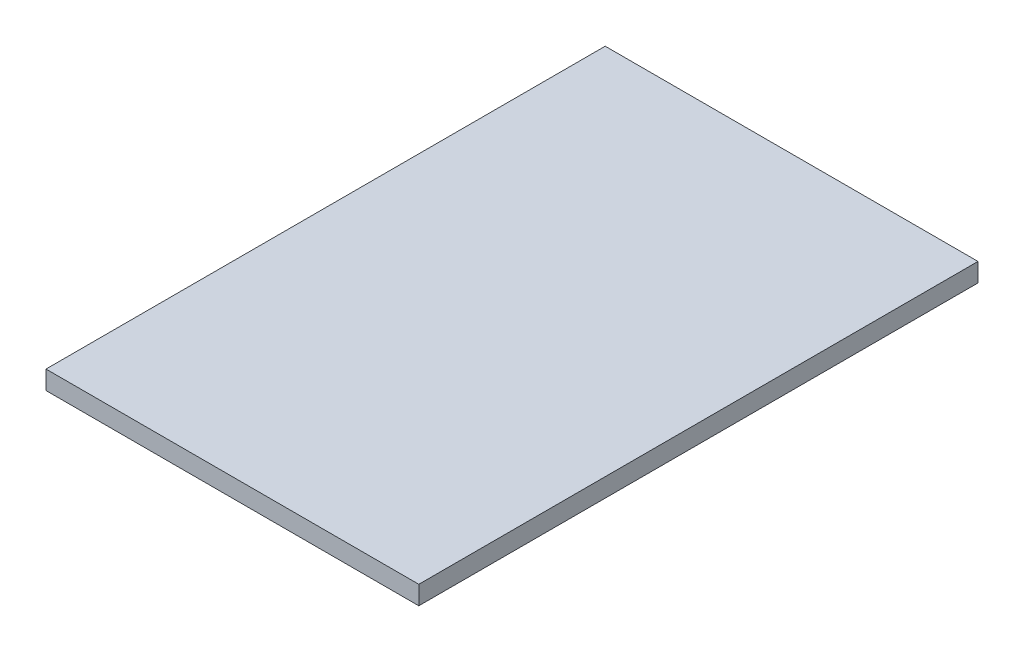
SolidWorks part; units mm, degrees
ref_plane "Front Plane" through (0, 0, 0) normal (0, 0, 1) x (1, 0, 0)
ref_plane "Top Plane" through (0, 0, 0) normal (0, 1, 0) x (1, 0, 0)
ref_plane "Right Plane" through (0, 0, 0) normal (1, 0, 0) x (0, 0, -1)
sketch "Sketch1" plane through (0, 0, 0) normal (0, 1, 0) x (1, 0, 0)
  line L1 (-100, 150) -> (100, 150)
  line L2 (-100, 150) -> (-100, -150)
  line L3 (-100, -150) -> (100, -150)
  line L4 (100, 150) -> (100, -150)
  line L5 (-100, 150) -> (100, -150) construction
  line L6 (-100, -150) -> (100, 150) construction
  point P0 (0, 0)
  dimension "D1" = 200
  dimension "D2" = 300
extrude "Boss-Extrude1" add sketch "Sketch1" along normal blind 10
